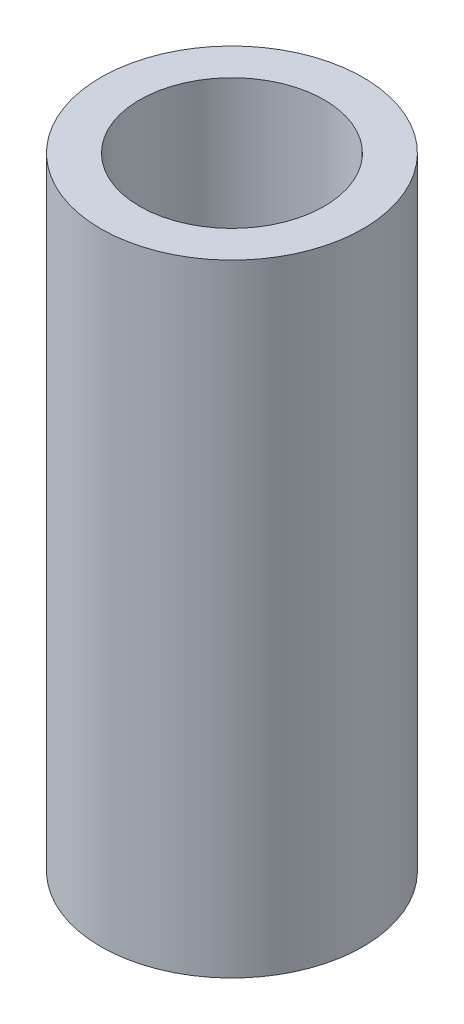
from build123d import *

# Parameters (mm, degrees)
SKETCH1_R      = 13.5
SKETCH1_R_2    = 9.5
EXTRUDE1_DEPTH = 64


with BuildPart() as part:
    # Sketch1 → Extrude1 (new body)
    with BuildSketch(Plane(origin=(0, 0, 0), x_dir=(1, 0, 0), z_dir=(0, 1, 0))):
        with Locations(Location((0, 0, 0), (0, 0, 270))):
            Circle(SKETCH1_R)
        with Locations(Location((0, 0, 0), (0, 0, 270))):
            Circle(SKETCH1_R_2, mode=Mode.SUBTRACT)
    extrude(amount=EXTRUDE1_DEPTH)


solid = part.part
